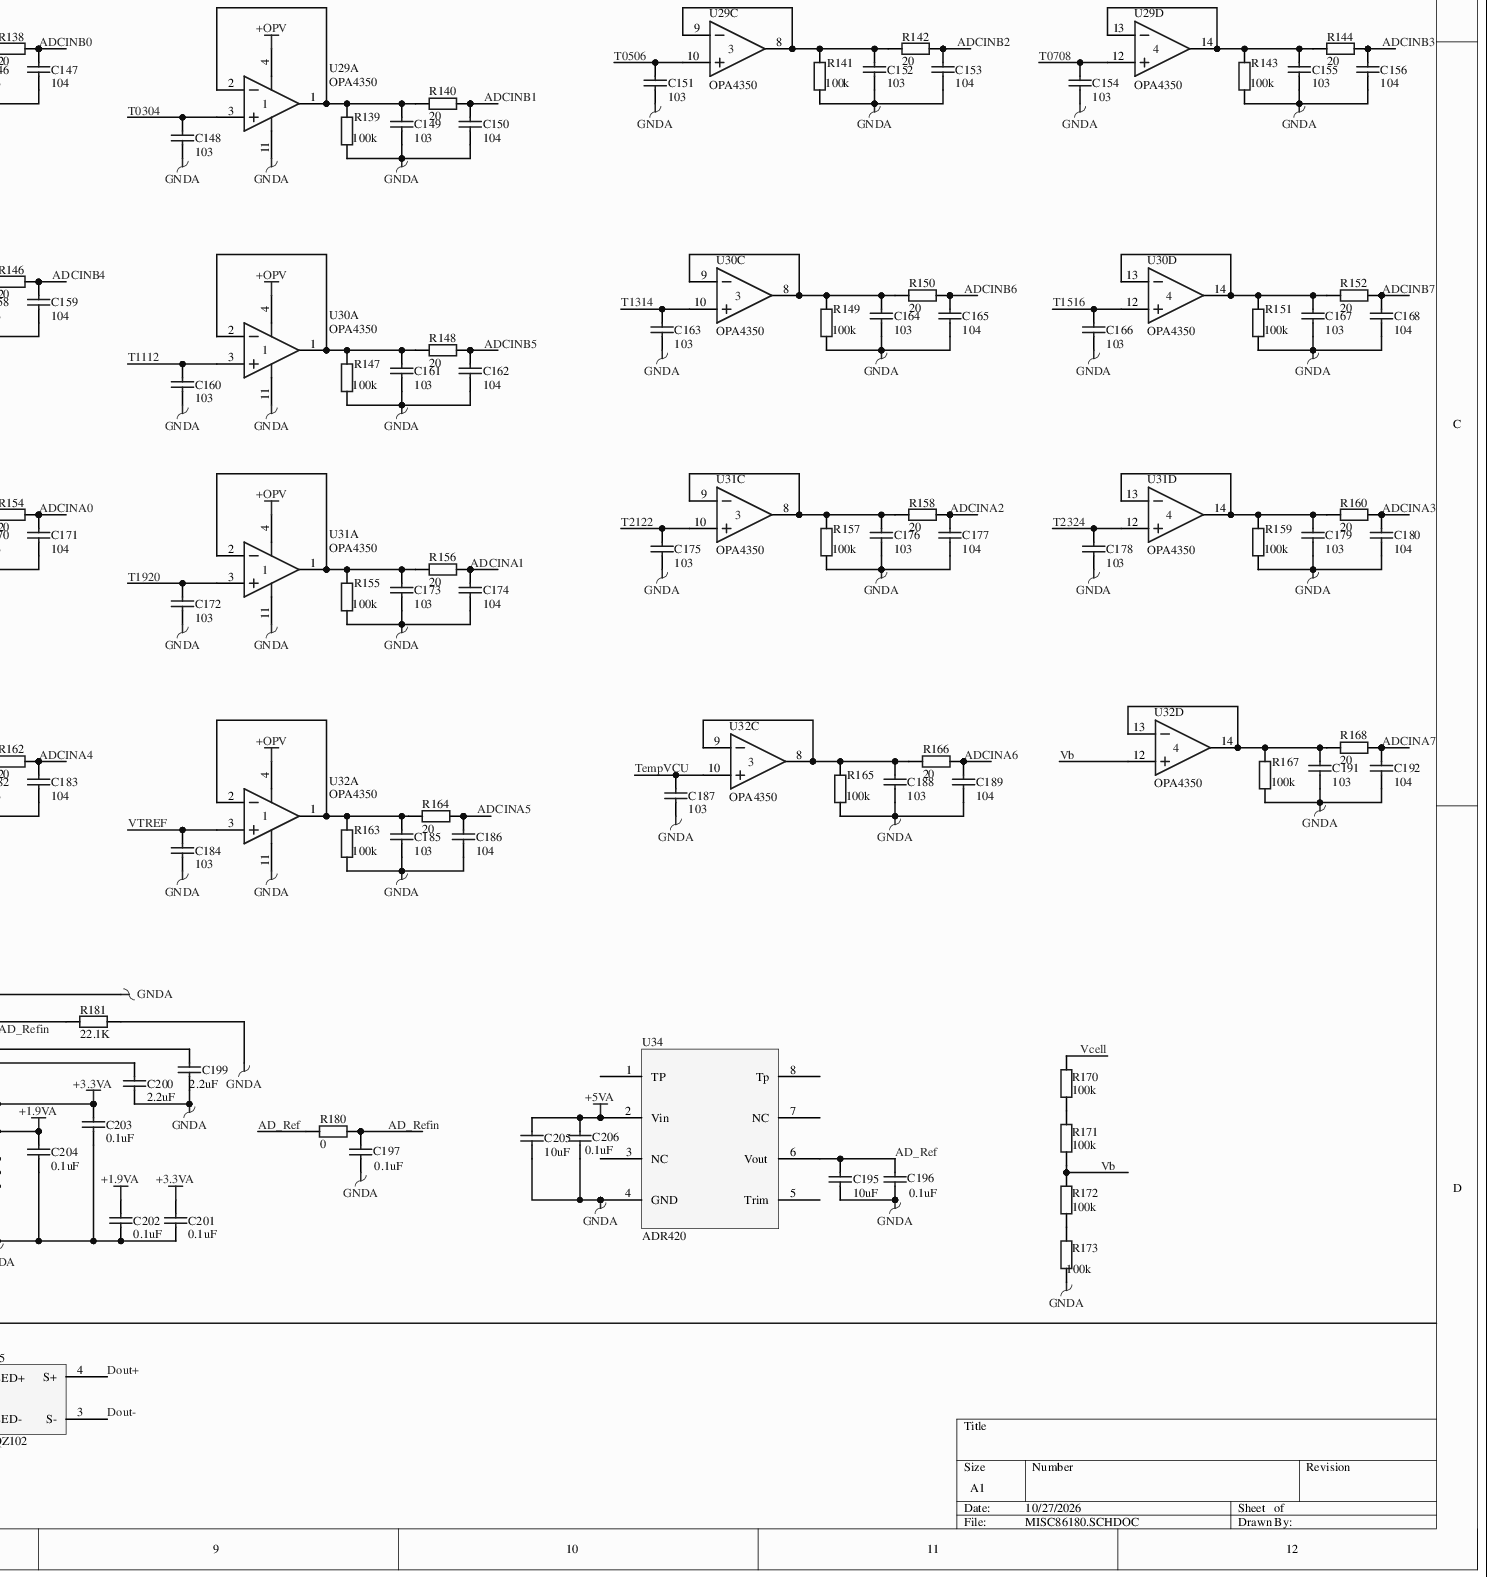
[diagram p0: MISC86180.SCHDOC, bottom right]
# Altium project MISC86180-9.PrjPCB (part 2 of 3)

## Sheet MISC86180.SCHDOC
size A1

### Parts
B1  BNX012H  [BNX012H]
C1  value 100uF  [TC7343-2917]  (hidden comment: Cap Pol3)
C2  value 47uF  [TC7343-2917]  (hidden comment: Cap Pol3)
C3  value 47uF  [TC7343-2917]  (hidden comment: Cap Pol3)
C4  value 0.1uF  [CR2012-0805]  (hidden comment: Cap)
C5  value 47uF  [TC7343-2917]  (hidden comment: Cap Pol3)
C6  value 47uF  [TC7343-2917]  (hidden comment: Cap Pol3)
C7  value 0.1uF  [CR2012-0805]  (hidden comment: Cap)
C8  value 47uF  [TC7343-2917]  (hidden comment: Cap Pol3)
C9  value 47uF  [TC7343-2917]  (hidden comment: Cap Pol3)
C10  value 0.1uF  [CR2012-0805]  (hidden comment: Cap)
C11  value 47uF  [TC7343-2917]  (hidden comment: Cap Pol3)
C12  value 0.1uF  [CR1608-0603]  (hidden comment: Cap)
C13  value 47uF  [TC7343-2917]  (hidden comment: Cap Pol3)
C14  value 0.1uF  [CR1608-0603]  (hidden comment: Cap)
C15  value 47uF  [TC7343-2917]  (hidden comment: Cap Pol3)
C16  value 0.1uF  [CR1608-0603]  (hidden comment: Cap)
C17  value 47uF  [TC7343-2917]  (hidden comment: Cap Pol3)
C18  value 0.1uF  [CR1608-0603]  (hidden comment: Cap)
C19  value 0.1uF  [CR1608-0603]  (hidden comment: Cap)
C20  value 0.1uF  [CR1608-0603]  (hidden comment: Cap)
C21  value 0.1uF  [CR1608-0603]  (hidden comment: Cap)
C22  value 0.1uF  [CR1608-0603]  (hidden comment: Cap)
C23  value 0.1uF  [CR1608-0603]  (hidden comment: Cap)
C24  value 0.1uF  [CR1608-0603]  (hidden comment: Cap)
C25  value 0.1uF  [CR1608-0603]  (hidden comment: Cap)
C26  value 0.1uF  [CR1608-0603]  (hidden comment: Cap)
C27  value 0.1uF  [CR1608-0603]  (hidden comment: Cap)
C28  value 0.1uF  [CR1608-0603]  (hidden comment: Cap)
C29  value 0.1uF  [CR1608-0603]  (hidden comment: Cap)
C30  value 0.1uF  [CR1608-0603]  (hidden comment: Cap)
C31  value 0.1uF  [CR1608-0603]  (hidden comment: Cap)
C32  value 0.1uF  [CR1608-0603]  (hidden comment: Cap)
C33  value 0.1uF  [CR1608-0603]  (hidden comment: Cap)
C34  value 0.1uF  [CR1608-0603]  (hidden comment: Cap)
C35  value 0.1uF  [CR1608-0603]  (hidden comment: Cap)
C36  value 0.1uF  [CR1608-0603]  (hidden comment: Cap)
C37  value 0.1uF  [CR1608-0603]  (hidden comment: Cap)
C38  value 0.1uF  [CR1608-0603]  (hidden comment: Cap)
C39  value 0.1uF  [CR1608-0603]  (hidden comment: Cap)
C40  value 0.1uF  [CR1608-0603]  (hidden comment: Cap)
C41  value 0.1uF  [CR1608-0603]  (hidden comment: Cap)
C42  value 0.1uF  [CR1608-0603]  (hidden comment: Cap)
C46  value 1uF  [1206]  (hidden comment: Cap)
C47  value 0.1uF  [CR1608-0603]  (hidden comment: Cap)
C48  value 0.001uF  [CR1608-0603]  (hidden comment: Cap)
C52  value 330PF  [CR1608-0603]  (hidden comment: Cap)
C53  value 0.1uF  [CR1608-0603]  (hidden comment: Cap)
C54  value 0.1uF  [CR1608-0603]  (hidden comment: Cap)
C55  value 24pF  [CR1608-0603]  (hidden comment: Cap)
C56  value 24pF  [CR1608-0603]  (hidden comment: Cap)
C57  value 0.1uF  [CR1608-0603]  (hidden comment: Cap)
C58  value 101  [CR1608-0603]  (hidden comment: Cap)
C59  value 101  [CR1608-0603]  (hidden comment: Cap)
C60  value 101  [CR1608-0603]  (hidden comment: Cap)
C61  value 101  [CR1608-0603]  (hidden comment: Cap)
C62  value 474  [CR1608-0603]  (hidden comment: Cap)
C63  value 684  [CR1608-0603]  (hidden comment: Cap)
C64  value 10uF  [CR3216-1206]  (hidden comment: Cap)
C65  value 0.1uF  [CR1608-0603]  (hidden comment: Cap)
C66  value 0.1uF  [CR1608-0603]  (hidden comment: Cap)
C67  value 0.1uF  [CR1608-0603]  (hidden comment: Cap)
C68  value 0.1uF  [CR1608-0603]  (hidden comment: Cap)
C69  value 0.1uF  [CR1608-0603]  (hidden comment: Cap)
C81  value 47uF  [TC7343-2917]  (hidden comment: Cap Pol3)
C82  value 0.1uF  [CR1608-0603]  (hidden comment: Cap)
C83  value 0.1uF  [CR1608-0603]  (hidden comment: Cap)
C84  value 0.1uF  [CR1608-0603]  (hidden comment: Cap)
C85  value 0.1uF  [CR1608-0603]  (hidden comment: Cap)
C86  value 0.1uF  [CR1608-0603]  (hidden comment: Cap)
C87  value 0.1uF  [CR1608-0603]  (hidden comment: Cap)
C88  value 0.1uF  [CR1608-0603]  (hidden comment: Cap)
C89  value 0.1uF  [CR1608-0603]  (hidden comment: Cap)
C90  value 0.1uF  [CR1608-0603]  (hidden comment: Cap)
C91  value 10uF  [CR3216-1206]  (hidden comment: Cap)
C92  value 0.1uF  [CR1608-0603]  (hidden comment: Cap)
C93  value 0.1uF  [CR1608-0603]  (hidden comment: Cap)
C94  value 0.1uF  [CR1608-0603]  (hidden comment: Cap)
C95  value 0.1uF  [CR1608-0603]  (hidden comment: Cap)
C96  value 0.1uF  [CR1608-0603]  (hidden comment: Cap)
C97  value 0.1uF  [CR1608-0603]  (hidden comment: Cap)
C98  value 0.1uF  [CR1608-0603]  (hidden comment: Cap)
C99  value 0.1uF  [CR1608-0603]  (hidden comment: Cap)
C100  value 0.1uF  [CR1608-0603]  (hidden comment: Cap)
C101  value 0.1uF  [CR1608-0603]  (hidden comment: Cap)
C102  value 0.1uF  [CR1608-0603]  (hidden comment: Cap)
C103  value 0.1uF  [CR1608-0603]  (hidden comment: Cap)
C104  value 0.1uF  [CR1608-0603]  (hidden comment: Cap)
C105  value 0.1uF  [CR1608-0603]  (hidden comment: Cap)
C106  value 0.1uF  [CR1608-0603]  (hidden comment: Cap)
C107  value 0.1uF  [CR1608-0603]  (hidden comment: Cap)
C108  value 0.1uF  [CR1608-0603]  (hidden comment: Cap)
C109  value 0.1uF  [CR1608-0603]  (hidden comment: Cap)
C110  value 0.1uF  [CR1608-0603]  (hidden comment: Cap)
C111  value 0.1uF  [CR1608-0603]  (hidden comment: Cap)
C112  value 0.1uF  [CR1608-0603]  (hidden comment: Cap)
C113  value 0.1uF  [CR1608-0603]  (hidden comment: Cap)
C114  value 0.1uF  [CR1608-0603]  (hidden comment: Cap)
C115  value 0.1uF  [CR1608-0603]  (hidden comment: Cap)
C116  value 0.1uF  [CR1608-0603]  (hidden comment: Cap)
C117  value 0.1uF  [CR1608-0603]  (hidden comment: Cap)
C118  value 0.1uF  [CR1608-0603]  (hidden comment: Cap)
C119  value 0.1uF  [CR1608-0603]  (hidden comment: Cap)
C120  value 0.1uF  [CR1608-0603]  (hidden comment: Cap)
C121  value 0.1uF  [CR1608-0603]  (hidden comment: Cap)
C122  value 0.1uF  [CR1608-0603]  (hidden comment: Cap)
C123  value 0.1uF  [CR1608-0603]  (hidden comment: Cap)
C124  value 0.1uF  [CR1608-0603]  (hidden comment: Cap)
C125  value 0.1uF  [CR2012-0805]  (hidden comment: Cap)
C126  value 0.1uF  [CR2012-0805]  (hidden comment: Cap)
C127  value 0.1uF  [CR2012-0805]  (hidden comment: Cap)
C128  value 0.1uF  [CR2012-0805]  (hidden comment: Cap)
C129  value 10uF  [CR3216-1206]  (hidden comment: Cap)
C130  value 10uF  [CR3216-1206]  (hidden comment: Cap)
C131  value 10uF  [CR3216-1206]  (hidden comment: Cap)
C132  value 10uF  [CR3216-1206]  (hidden comment: Cap)
C133  value 10uF  [CR3216-1206]  (hidden comment: Cap)
C134  value 10uF  [CR3216-1206]  (hidden comment: Cap)
C135  value 10uF  [CR3216-1206]  (hidden comment: Cap)
C136  value 0.1uF  [CR1608-0603]  (hidden comment: Cap)
C137  value 0.1uF  [CR1608-0603]  (hidden comment: Cap)
C138  value 0.1uF  [CR1608-0603]  (hidden comment: Cap)
C139  value 0.1uF  [CR1608-0603]  (hidden comment: Cap)
C140  value 0.1uF  [CR1608-0603]  (hidden comment: Cap)
C141  value 0.1uF  [CR1608-0603]  (hidden comment: Cap)
C142  value 0.1uF  [CR1608-0603]  (hidden comment: Cap)
C143  value 10uF  [CR3216-1206]  (hidden comment: Cap)
C144  value 0.1uF  [CR1608-0603]  (hidden comment: Cap)
C145  value 103  [CR1608-0603]  (hidden comment: Cap)
C146  value 103  [CR1608-0603]  (hidden comment: Cap)
C147  value 104  [CR1608-0603]  (hidden comment: Cap)
C148  value 103  [CR1608-0603]  (hidden comment: Cap)
C149  value 103  [CR1608-0603]  (hidden comment: Cap)
C150  value 104  [CR1608-0603]  (hidden comment: Cap)
C151  value 103  [CR1608-0603]  (hidden comment: Cap)
C152  value 103  [CR1608-0603]  (hidden comment: Cap)
C153  value 104  [CR1608-0603]  (hidden comment: Cap)
C154  value 103  [CR1608-0603]  (hidden comment: Cap)
C155  value 103  [CR1608-0603]  (hidden comment: Cap)
C156  value 104  [CR1608-0603]  (hidden comment: Cap)
C157  value 103  [CR1608-0603]  (hidden comment: Cap)
C158  value 103  [CR1608-0603]  (hidden comment: Cap)
C159  value 104  [CR1608-0603]  (hidden comment: Cap)
C160  value 103  [CR1608-0603]  (hidden comment: Cap)
C161  value 103  [CR1608-0603]  (hidden comment: Cap)
C162  value 104  [CR1608-0603]  (hidden comment: Cap)
C163  value 103  [CR1608-0603]  (hidden comment: Cap)
C164  value 103  [CR1608-0603]  (hidden comment: Cap)
C165  value 104  [CR1608-0603]  (hidden comment: Cap)
C166  value 103  [CR1608-0603]  (hidden comment: Cap)
C167  value 103  [CR1608-0603]  (hidden comment: Cap)
C168  value 104  [CR1608-0603]  (hidden comment: Cap)
C169  value 103  [CR1608-0603]  (hidden comment: Cap)
C170  value 103  [CR1608-0603]  (hidden comment: Cap)
C171  value 104  [CR1608-0603]  (hidden comment: Cap)
C172  value 103  [CR1608-0603]  (hidden comment: Cap)
C173  value 103  [CR1608-0603]  (hidden comment: Cap)
C174  value 104  [CR1608-0603]  (hidden comment: Cap)
C175  value 103  [CR1608-0603]  (hidden comment: Cap)
C176  value 103  [CR1608-0603]  (hidden comment: Cap)
C177  value 104  [CR1608-0603]  (hidden comment: Cap)
C178  value 103  [CR1608-0603]  (hidden comment: Cap)
C179  value 103  [CR1608-0603]  (hidden comment: Cap)
C180  value 104  [CR1608-0603]  (hidden comment: Cap)
C181  value 103  [CR1608-0603]  (hidden comment: Cap)
C182  value 103  [CR1608-0603]  (hidden comment: Cap)
C183  value 104  [CR1608-0603]  (hidden comment: Cap)
C184  value 103  [CR1608-0603]  (hidden comment: Cap)
C185  value 103  [CR1608-0603]  (hidden comment: Cap)
C186  value 104  [CR1608-0603]  (hidden comment: Cap)
C187  value 103  [CR1608-0603]  (hidden comment: Cap)
C188  value 103  [CR1608-0603]  (hidden comment: Cap)
C189  value 104  [CR1608-0603]  (hidden comment: Cap)
C191  value 103  [CR1608-0603]  (hidden comment: Cap)
C192  value 104  [CR1608-0603]  (hidden comment: Cap)
C195  value 10uF  [CR3216-1206]  (hidden comment: Cap)
C196  value 0.1uF  [CR1608-0603]  (hidden comment: Cap)
C197  value 0.1uF  [CR1608-0603]  (hidden comment: Cap)
C199  value 2.2uF  [CR1608-0603]  (hidden comment: Cap)
C200  value 2.2uF  [CR1608-0603]  (hidden comment: Cap)
C201  value 0.1uF  [CR1608-0603]  (hidden comment: Cap)
C202  value 0.1uF  [CR1608-0603]  (hidden comment: Cap)
C203  value 0.1uF  [CR1608-0603]  (hidden comment: Cap)
C204  value 0.1uF  [CR1608-0603]  (hidden comment: Cap)
C205  value 10uF  [CR3216-1206]  (hidden comment: Cap)
C206  value 0.1uF  [CR1608-0603]  (hidden comment: Cap)
C208  value 10uF  [CR3216-1206]  (hidden comment: Cap)
C209  value 0.1uF  [CR1608-0603]  (hidden comment: Cap)
D1  RED  [CR2012-0805]
D2  RED  [CR2012-0805]
D3  GREEN  [CR2012-0805]
D4  GREEN  [CR2012-0805]
D5  BLUE  [CR2012-0805]
D6  BLUE  [CR2012-0805]
D7  BLUE  [CR2012-0805]
D8  BLUE  [CR2012-0805]
D9  BLUE  [CR2012-0805]
D10  value BLUE  [CR2012-0805]  (hidden comment: RED)
DZ1  SMBJ8.5CA  [AK_1B]
DZ2  SMBJ8.5CA  [AK_1B]
F1  value 500mA  [CR6332-2512]  (hidden comment: Res2)
F2  value 500mA  [CR6332-2512]  (hidden comment: Res2)
F3  value 500mA  [CR6332-2512]  (hidden comment: Res2)
F4  value 500mA  [CR6332-2512]  (hidden comment: Res2)
F5  value 500mA  [CR6332-2512]  (hidden comment: Res2)
F6  value 500mA  [CR6332-2512]  (hidden comment: Res2)
F7  value 500mA  [CR6332-2512]  (hidden comment: Res2)
F8  value 500mA  [CR6332-2512]  (hidden comment: Res2)
F9  value 500mA  [CR6332-2512]  (hidden comment: Res2)
F10  value 500mA  [CR6332-2512]  (hidden comment: Res2)
F11  value 500mA  [CR6332-2512]  (hidden comment: Res2)
F12  value 500mA  [CR6332-2512]  (hidden comment: Res2)
F13  value 500mA  [CR6332-2512]  (hidden comment: Res2)
F14  value 500mA  [CR6332-2512]  (hidden comment: Res2)
F15  value 500mA  [CR6332-2512]  (hidden comment: Res2)
F16  value 500mA  [CR6332-2512]  (hidden comment: Res2)
F17  value 500mA  [CR6332-2512]  (hidden comment: Res2)
F18  value 500mA  [CR6332-2512]  (hidden comment: Res2)
F19  value 500mA  [CR6332-2512]  (hidden comment: Res2)
F20  value 500mA  [CR6332-2512]  (hidden comment: Res2)
F21  value 500mA  [CR6332-2512]  (hidden comment: Res2)
F22  value 500mA  [CR6332-2512]  (hidden comment: Res2)
F23  value 500mA  [CR6332-2512]  (hidden comment: Res2)
F24  value 500mA  [CR6332-2512]  (hidden comment: Res2)
F25  value 500mA  [CR6332-2512]  (hidden comment: Res2)
F26  value 500mA  [CR6332-2512]  (hidden comment: Res2)
F27  value 500mA  [CR6332-2512]  (hidden comment: Res2)
F28  value 500mA  [CR6332-2512]  (hidden comment: Res2)
F29  value 500mA  [CR6332-2512]  (hidden comment: Res2)
F30  value 500mA  [CR6332-2512]  (hidden comment: Res2)
F31  value 500mA  [CR6332-2512]  (hidden comment: Res2)
F32  value 500mA  [CR6332-2512]  (hidden comment: Res2)
F33  value 500mA  [CR6332-2512]  (hidden comment: Res2)
F34  value 500mA  [CR6332-2512]  (hidden comment: Res2)
F35  value 500mA  [CR6332-2512]  (hidden comment: Res2)
F36  value 500mA  [CR6332-2512]  (hidden comment: Res2)
F37  value 500mA  [CR6332-2512]  (hidden comment: Res2)
F38  value 500mA  [CR6332-2512]  (hidden comment: Res2)
F39  value 500mA  [CR6332-2512]  (hidden comment: Res2)
F40  value 500mA  [CR6332-2512]  (hidden comment: Res2)
F41  value 500mA  [CR6332-2512]  (hidden comment: Res2)
F42  value 500mA  [CR6332-2512]  (hidden comment: Res2)
F43  value 500mA  [CR6332-2512]  (hidden comment: Res2)
F44  value 500mA  [CR6332-2512]  (hidden comment: Res2)
F45  value 500mA  [CR6332-2512]  (hidden comment: Res2)
F46  value 500mA  [CR6332-2512]  (hidden comment: Res2)
F47  value 500mA  [CR6332-2512]  (hidden comment: Res2)
F48  value 500mA  [CR6332-2512]  (hidden comment: Res2)
F49  2.6A  [FUSE]
J1  JTAG_335  [JTAG14]
J2  Header 4  [HDR1X4]
J3  JTAG_CPLD  [HDR2X5]
JC1  AMP-36P  [36P]
JC2  AMP-28P  [28P]
L1  value BLM21PG221SH  [INDC2012-0805]  (hidden comment: Inductor)
L2  value 4.7uH  [CR3225-1210]  (hidden comment: Inductor)
L3  value 4.7uH  [CR3225-1210]  (hidden comment: Inductor)
R1  value 4.7k  [CR1608-0603]  (hidden comment: Res2)
R2  value 4.7k  [CR1608-0603]  (hidden comment: Res2)
R3  value 18.2K  [CR2012-0805]  (hidden comment: Res2)
R4  value 30.1K  [CR2012-0805]  (hidden comment: Res2)
R5  value 470  [CR1608-0603]  (hidden comment: Res2)
R6  value 470  [CR1608-0603]  (hidden comment: Res2)
R7  value 470  [CR1608-0603]  (hidden comment: Res2)
R8  value 4.7K  [CR1608-0603]  (hidden comment: Res2)
R9  value 1K  [CR1608-0603]  (hidden comment: Res2)
R10  value 1K  [CR1608-0603]  (hidden comment: Res2)
R11  value 1K  [CR1608-0603]  (hidden comment: Res2)
R12  value 1K  [CR1608-0603]  (hidden comment: Res2)
R13  value 10k  [CR1608-0603]  (hidden comment: Res2)
R14  value 20k  [CR1608-0603]  (hidden comment: Res2)
R17  value 60  [CR2012-0805]  (hidden comment: Res2)
R18  value 60  [CR2012-0805]  (hidden comment: Res2)
R19  value 1  [CR2012-0805]  (hidden comment: Res2)
R20  value 10k  [CR1608-0603]  (hidden comment: Res2)
R21  value 1k  [CR1608-0603]  (hidden comment: Res2)
R22  value 470  [CR1608-0603]  (hidden comment: Res2)
R23  value 1k  [CR1608-0603]  (hidden comment: Res2)
R24  value 470  [CR1608-0603]  (hidden comment: Res2)
R33  value 510  [CR2012-0805]  (hidden comment: Res2)
R34  value 510  [CR2012-0805]  (hidden comment: Res2)
R35  value 510  [CR2012-0805]  (hidden comment: Res2)
R36  value 510  [CR2012-0805]  (hidden comment: Res2)
R37  value 510  [CR2012-0805]  (hidden comment: Res2)
R38  value 510  [CR2012-0805]  (hidden comment: Res2)
R41  value 510  [CR2012-0805]  (hidden comment: Res2)
R42  value 510  [CR2012-0805]  (hidden comment: Res2)
R43  value 510  [CR2012-0805]  (hidden comment: Res2)
R44  value 510  [CR2012-0805]  (hidden comment: Res2)
R45  value 510  [CR2012-0805]  (hidden comment: Res2)
R46  value 510  [CR2012-0805]  (hidden comment: Res2)
R47  value 510  [CR2012-0805]  (hidden comment: Res2)
R48  value 510  [CR2012-0805]  (hidden comment: Res2)
R49  value 510  [CR2012-0805]  (hidden comment: Res2)
R50  value 510  [CR2012-0805]  (hidden comment: Res2)
R51  value 510  [CR2012-0805]  (hidden comment: Res2)
R52  value 510  [CR2012-0805]  (hidden comment: Res2)
R53  value 510  [CR2012-0805]  (hidden comment: Res2)
R54  value 510  [CR2012-0805]  (hidden comment: Res2)
R55  value 510  [CR2012-0805]  (hidden comment: Res2)
R56  value 510  [CR2012-0805]  (hidden comment: Res2)
R57  value 510  [CR2012-0805]  (hidden comment: Res2)
R58  value 510  [CR2012-0805]  (hidden comment: Res2)
R59  value 510  [CR2012-0805]  (hidden comment: Res2)
R60  value 510  [CR2012-0805]  (hidden comment: Res2)
R61  value 510  [CR2012-0805]  (hidden comment: Res2)
R62  value 510  [CR2012-0805]  (hidden comment: Res2)
R63  value 510  [CR2012-0805]  (hidden comment: Res2)
R64  value 510  [CR2012-0805]  (hidden comment: Res2)
R65  value 510  [CR2012-0805]  (hidden comment: Res2)
R66  value 510  [CR2012-0805]  (hidden comment: Res2)
R67  value 510  [CR2012-0805]  (hidden comment: Res2)
R68  value 510  [CR2012-0805]  (hidden comment: Res2)
R69  value 510  [CR2012-0805]  (hidden comment: Res2)
R70  value 510  [CR2012-0805]  (hidden comment: Res2)
R71  value 510  [CR2012-0805]  (hidden comment: Res2)
R72  value 510  [CR2012-0805]  (hidden comment: Res2)
R73  value 510  [CR2012-0805]  (hidden comment: Res2)
R74  value 510  [CR2012-0805]  (hidden comment: Res2)
R75  value 510  [CR2012-0805]  (hidden comment: Res2)
R76  value 510  [CR2012-0805]  (hidden comment: Res2)
R77  value 510  [CR2012-0805]  (hidden comment: Res2)
R78  value 510  [CR2012-0805]  (hidden comment: Res2)
R79  value 510  [CR2012-0805]  (hidden comment: Res2)
R80  value 510  [CR2012-0805]  (hidden comment: Res2)
R81  value 510  [CR2012-0805]  (hidden comment: Res2)
R82  value 510  [CR2012-0805]  (hidden comment: Res2)
R83  value 10k  [CR1608-0603]  (hidden comment: Res2)
R84  value 10k  [CR1608-0603]  (hidden comment: Res2)
R85  value 10k  [CR1608-0603]  (hidden comment: Res2)
R86  value 4.7k  [CR1608-0603]  (hidden comment: Res2)
R87  value 1k  [CR1608-0603]  (hidden comment: Res2)
R88  value 4.7k  [CR1608-0603]  (hidden comment: Res2)
R89  value 1k  [CR1608-0603]  (hidden comment: Res2)
R90  value 4.7k  [CR1608-0603]  (hidden comment: Res2)
R91  value 1k  [CR1608-0603]  (hidden comment: Res2)
R92  value 4.7k  [CR1608-0603]  (hidden comment: Res2)
R93  value 1k  [CR1608-0603]  (hidden comment: Res2)
R94  value 1k  [CR1608-0603]  (hidden comment: Res2)
R95  value 1k  [CR1608-0603]  (hidden comment: Res2)
R96  value 1k  [CR1608-0603]  (hidden comment: Res2)
R97  value 1k  [CR1608-0603]  (hidden comment: Res2)
R98  value 1k  [CR1608-0603]  (hidden comment: Res2)
R99  value 1k  [CR1608-0603]  (hidden comment: Res2)
R100  value 1k  [CR1608-0603]  (hidden comment: Res2)
R101  value 1k  [CR1608-0603]  (hidden comment: Res2)
R102  value 1k  [CR1608-0603]  (hidden comment: Res2)
R103  value 1k  [CR1608-0603]  (hidden comment: Res2)
R104  value 200  [CR2012-0805]  (hidden comment: Res2)
R105  value 4.7k  [CR1608-0603]  (hidden comment: Res2)
R106  value 10k  [CR2012-0805]  (hidden comment: Res2)
R107  value 10k  [CR2012-0805]  (hidden comment: Res2)
R108  value 10k  [CR2012-0805]  (hidden comment: Res2)
R109  value 10k  [CR2012-0805]  (hidden comment: Res2)
R110  value 10k  [CR2012-0805]  (hidden comment: Res2)
R111  value 10k  [CR2012-0805]  (hidden comment: Res2)
R112  value 10k  [CR2012-0805]  (hidden comment: Res2)
R113  value 10k  [CR2012-0805]  (hidden comment: Res2)
R114  value 10k  [CR2012-0805]  (hidden comment: Res2)
R115  value 10k  [CR2012-0805]  (hidden comment: Res2)
R116  value 10k  [CR2012-0805]  (hidden comment: Res2)
R117  value 10k  [CR2012-0805]  (hidden comment: Res2)
R118  value 10k  [CR2012-0805]  (hidden comment: Res2)
R119  value 10k  [CR2012-0805]  (hidden comment: Res2)
R120  value 10k  [CR2012-0805]  (hidden comment: Res2)
R121  value 10k  [CR2012-0805]  (hidden comment: Res2)
R122  value 10k  [CR2012-0805]  (hidden comment: Res2)
R123  value 10k  [CR2012-0805]  (hidden comment: Res2)
R124  value 10k  [CR2012-0805]  (hidden comment: Res2)
R125  value 10k  [CR2012-0805]  (hidden comment: Res2)
R126  value 10k  [CR2012-0805]  (hidden comment: Res2)
R127  value 10k  [CR2012-0805]  (hidden comment: Res2)
R128  value 10k  [CR2012-0805]  (hidden comment: Res2)
R129  value 10k  [CR2012-0805]  (hidden comment: Res2)
R130  value 10k  [CR2012-0805]  (hidden comment: Res2)
R131  value 10k  [CR2012-0805]  (hidden comment: Res2)
R132  value 10k  [CR2012-0805]  (hidden comment: Res2)
R133  value 10k  [CR2012-0805]  (hidden comment: Res2)
R134  value 10k  [CR2012-0805]  (hidden comment: Res2)
R136  value 0  [CR2012-0805]  (hidden comment: Res2)
R137  value 100k  [CR1608-0603]  (hidden comment: Res2)
R138  value 20  [CR1608-0603]  (hidden comment: Res2)
R139  value 100k  [CR1608-0603]  (hidden comment: Res2)
R140  value 20  [CR1608-0603]  (hidden comment: Res2)
R141  value 100k  [CR1608-0603]  (hidden comment: Res2)
R142  value 20  [CR1608-0603]  (hidden comment: Res2)
R143  value 100k  [CR1608-0603]  (hidden comment: Res2)
R144  value 20  [CR1608-0603]  (hidden comment: Res2)
R145  value 100k  [CR1608-0603]  (hidden comment: Res2)
R146  value 20  [CR1608-0603]  (hidden comment: Res2)
R147  value 100k  [CR1608-0603]  (hidden comment: Res2)
R148  value 20  [CR1608-0603]  (hidden comment: Res2)
R149  value 100k  [CR1608-0603]  (hidden comment: Res2)
R150  value 20  [CR1608-0603]  (hidden comment: Res2)
R151  value 100k  [CR1608-0603]  (hidden comment: Res2)
R152  value 20  [CR1608-0603]  (hidden comment: Res2)
R153  value 100k  [CR1608-0603]  (hidden comment: Res2)
R154  value 20  [CR1608-0603]  (hidden comment: Res2)
R155  value 100k  [CR1608-0603]  (hidden comment: Res2)
R156  value 20  [CR1608-0603]  (hidden comment: Res2)
R157  value 100k  [CR1608-0603]  (hidden comment: Res2)
R158  value 20  [CR1608-0603]  (hidden comment: Res2)
R159  value 100k  [CR1608-0603]  (hidden comment: Res2)
R160  value 20  [CR1608-0603]  (hidden comment: Res2)
R161  value 100k  [CR1608-0603]  (hidden comment: Res2)
R162  value 20  [CR1608-0603]  (hidden comment: Res2)
R163  value 100k  [CR1608-0603]  (hidden comment: Res2)
R164  value 20  [CR1608-0603]  (hidden comment: Res2)
R165  value 100k  [CR1608-0603]  (hidden comment: Res2)
R166  value 20  [CR1608-0603]  (hidden comment: Res2)
R167  value 100k  [CR1608-0603]  (hidden comment: Res2)
R168  value 20  [CR1608-0603]  (hidden comment: Res2)
R170  value 100k  [CR2012-0805]  (hidden comment: Res2)
R171  value 100k  [CR2012-0805]  (hidden comment: Res2)
R172  value 100k  [CR2012-0805]  (hidden comment: Res2)
R173  value 100k  [CR2012-0805]  (hidden comment: Res2)
R180  value 0  [CR2012-0805]  (hidden comment: Res2)
R181  value 22.1K  [CR1608-0603]  (hidden comment: Res2)
S1  AQW214  [AQW214]
S2  AQW214  [AQW214]
S3  AQW214  [AQW214]
S4  AQW214  [AQW214]
S5  AQW214  [AQW214]
S6  AQW214  [AQW214]
S7  AQW214  [AQW214]
S8  AQW214  [AQW214]
S9  AQW214  [AQW214]
S10  AQW214  [AQW214]
S11  AQW214  [AQW214]
S12  AQW214  [AQW214]
S13  AQW214  [AQW214]
S14  AQW214  [AQW214]
S15  AQW214  [AQW214]
S16  AQW214  [AQW214]
S17  AQW214  [AQW214]
S18  AQW214  [AQW214]
S19  AQW214  [AQW214]
S20  AQW214  [AQW214]
S21  AQW214  [AQW214]
S22  AQW214  [AQW214]
S23  AQW214  [AQW214]
S24  AQW214  [AQW214]
SW1  SW-PB  [SW_RESET]
TVS1  1.5KE30A  [SB560]
U1  1205  [DCDC_5W]
U2  1205  [DCDC_5W]
U3  1205  [DCDC_5W]
U4  TPS75733  [75733]
U5  TPS76801Q  [D008]
U6  TPS75733  [75733]
U7  TPS75733  [75733]
U8  TPS3823-33  [DBV005]
U9  TMS320F283XXPGF_23  [QFP176NEW]  (parts A,B,C,D of 4)
U10  SN74CBTD3384DBLE  [DBQ024]
U11  ZJYS-81R5-2PL  [ZJYS]
U13  SN65HVD251  [D008]
U15  HCPL063  [SO-G8]
U16  HCPL063  [SO-G8]
U19  EPM240T100C5N  [TQFP100]  (parts A,B,C of 3)
U20  SN74CBTD3384DBLE  [DBQ024]
U21  SN74LVC4245PW  [WSO24]
U22  SN74LVC4245PW  [WSO24]
U23  SN74LVC4245PW  [WSO24]
U24  SN74LVC4245PW  [WSO24]
U25  MAX4619  [SO16]
U26  MAX4619  [SO16]
U27  MAX4619  [SO16]
U28  MAX4619  [SO16]
U29  OPA4350  [751A-02]  (parts A,B,C,D of 4)
U30  OPA4350  [751A-02]  (parts A,B,C,D of 4)
U31  OPA4350  [751A-02]  (parts A,B,C,D of 4)
U32  OPA4350  [751A-02]  (parts A,B,C,D of 4)
U34  ADR420  [SO-G8]
U35  AQZ102  [AQZ102]
Y1  30M  [Oscillator]